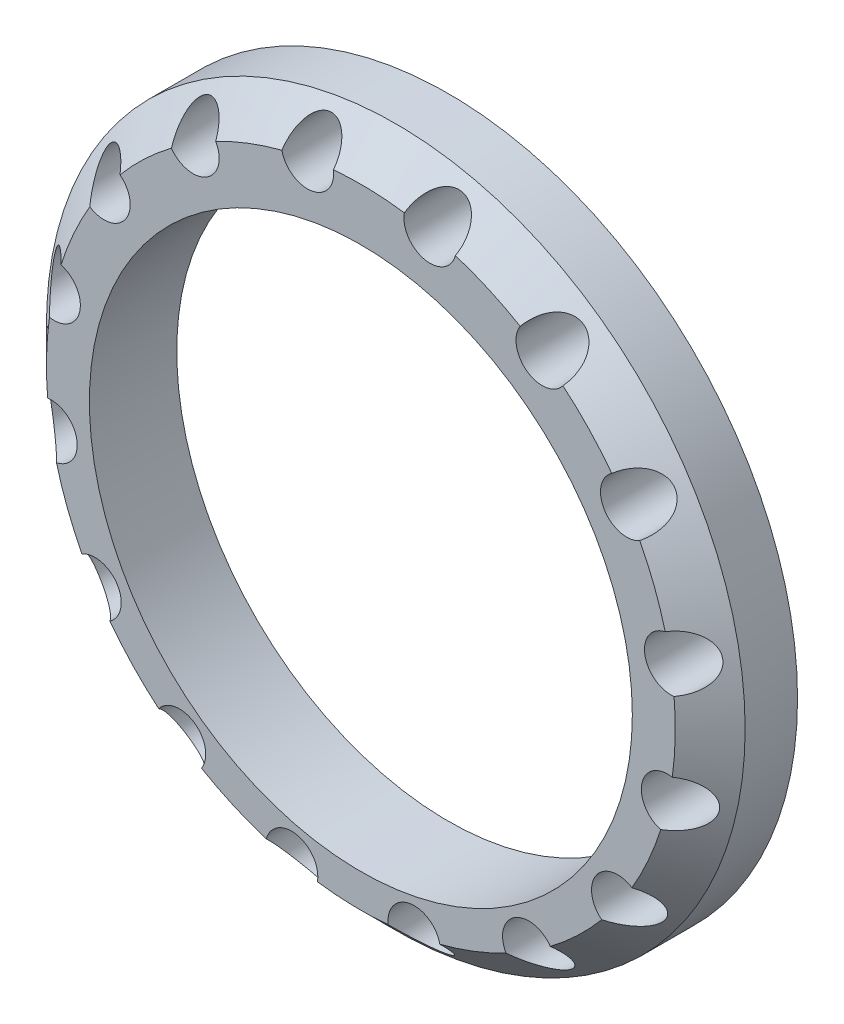
SolidWorks part; units mm, degrees
ref_plane "Front Plane" through (0, 0, 0) normal (0, 0, 1) x (1, 0, 0)
ref_plane "Top Plane" through (0, 0, 0) normal (0, 1, 0) x (1, 0, 0)
ref_plane "Right Plane" through (0, 0, 0) normal (1, 0, 0) x (0, 0, -1)
sketch "Sketch1" plane through (0, 0, 0) normal (0, 0, 1) x (1, 0, 0)
  line L0 (20, 70.8305) -> (20, 40.8305) construction
  circle A0 centre (20, 55.8305) radius 20
  circle A1 centre (20, 55.2893) radius 15.5412
extrude "Boss-Extrude1" add sketch "Sketch1" along normal blind 5
chamfer "Chamfer1" distance 2 angle 45 1 edges at (40, 55.8305, 5)
sketch "Sketch2" plane through (0, 0, 5) normal (0, 0, 1) x (1, 0, 0)
  line L0 (20, 70.8305) -> (20, 40.8305) construction
  circle A0 centre (20, 55.8305) radius 18 construction
  circle A2 centre (10.3884, 71.0495) radius 1.5
  circle A4 centre (16.9441, 73.5692) radius 1.5
  circle A5 centre (23.965, 73.3884) radius 1.5
  circle A6 centre (30.3823, 70.5345) radius 1.5
  circle A7 centre (35.219, 65.4421) radius 1.5
  circle A8 centre (37.7387, 58.8864) radius 1.5
  circle A9 centre (37.5579, 51.8655) radius 1.5
  circle A10 centre (34.704, 45.4482) radius 1.5
  circle A11 centre (29.6116, 40.6115) radius 1.5
  circle A12 centre (23.0559, 38.0918) radius 1.5
  circle A13 centre (16.035, 38.2726) radius 1.5
  circle A14 centre (9.6177, 41.1265) radius 1.5
  circle A15 centre (4.781, 46.2189) radius 1.5
  circle A16 centre (2.2613, 52.7746) radius 1.5
  circle A17 centre (2.4421, 59.7955) radius 1.5
  circle A18 centre (5.296, 66.2128) radius 1.5
  dimension "D1" = 36
  dimension "D2" = 3
  dimension "D3" = 16
extrude "Cut-Extrude1" cut sketch "Sketch2" against normal through all
